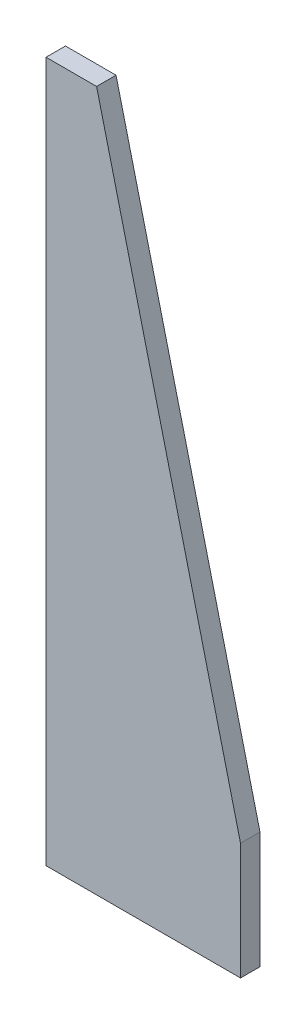
SolidWorks part; units mm, degrees
ref_plane "Front Plane" through (0, 0, 0) normal (0, 0, 1) x (1, 0, 0)
ref_plane "Top Plane" through (0, 0, 0) normal (0, 1, 0) x (1, 0, 0)
ref_plane "Right Plane" through (0, 0, 0) normal (1, 0, 0) x (0, 0, -1)
other "Configuration Table"
sketch "Sketch1" plane through (0, 0, 0) normal (0, 0, 1) x (1, 0, 0)
  line L0 (0, 0) -> (100, 0)
  line L1 (100, 0) -> (100, 60)
  line L2 (100, 60) -> (26, 360)
  line L3 (26, 360) -> (0, 360)
  line L4 (0, 360) -> (0, 0)
  dimension "D1" = 100
  dimension "D2" = 360
  dimension "D3" = 60
  dimension "D4" = 26
extrude "Boss-Extrude1" add sketch "Sketch1" along normal blind 10
